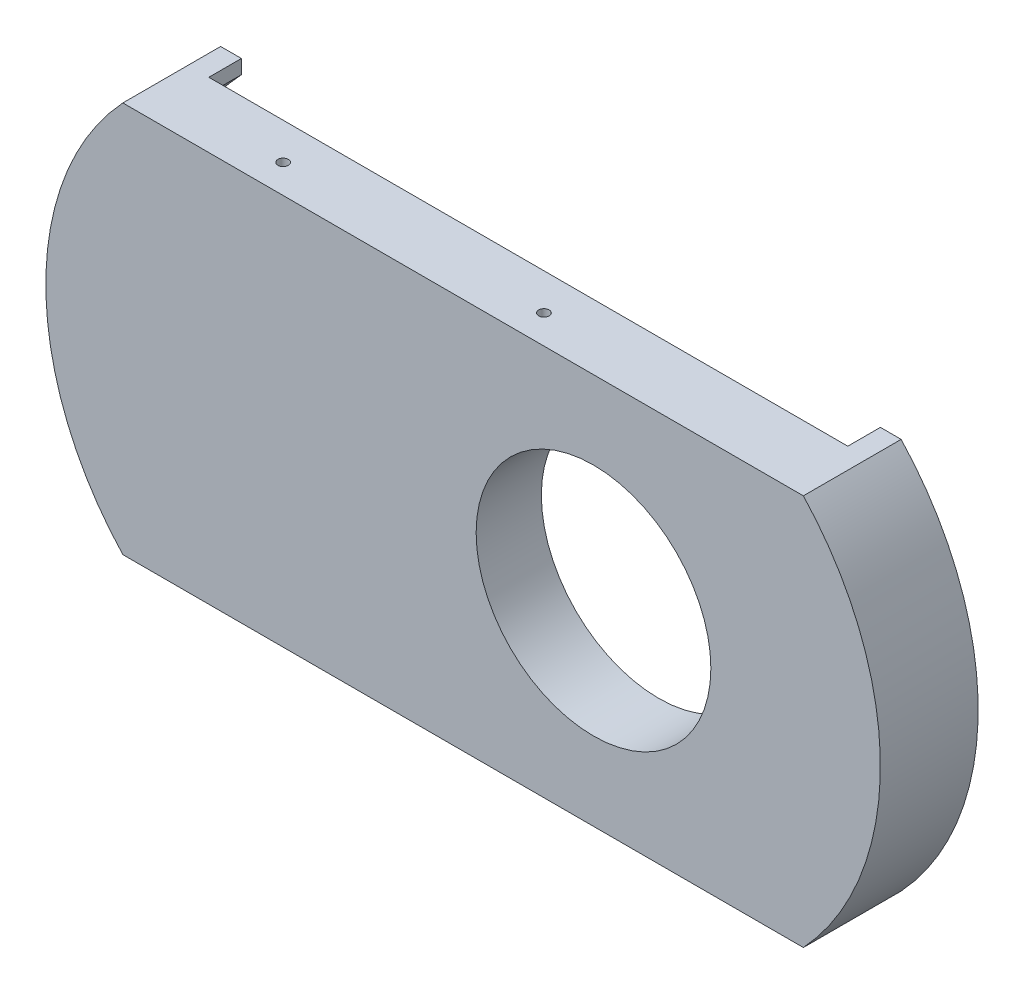
from build123d import *

# Parameters (mm, degrees)
SKETCH1_R                      = 2
BOSS_EXTRUDE1_DEPTH            = 5
SKETCH2_R                      = 8.5
CUT_EXTRUDE1_DEPTH             = 2
CUT_EXTRUDE2_REACH             = 37.693
SKETCH3_R                      = 9
BOSS_EXTRUDE2_START            = 2.5
BOSS_EXTRUDE2_DEPTH            = 2.5
SKETCH5_W                      = 49
SKETCH5_H                      = 36.444930448
CUT_EXTRUDE3_DEPTH             = 11.5
F_0_8_0_8_DIAMETER_HOLE1_D     = 0.8
F_0_8_0_8_DIAMETER_HOLE1_DEPTH = 1
F_0_8_0_8_DIAMETER_HOLE1_TIP   = 0.240344248
SKETCH8_R                      = 2
BOSS_EXTRUDE3_DEPTH            = 3
F_0_8_0_8_DIAMETER_HOLE2_D     = 0.8
F_0_8_0_8_DIAMETER_HOLE2_DEPTH = 1
F_0_8_0_8_DIAMETER_HOLE2_TIP   = 0.240344248


with BuildPart() as part:
    # Sketch1 → Boss-Extrude1 (new body)
    with BuildSketch(Plane.XY):
        with BuildLine():
            Line((-26.093476939, 15), (26.093476939, 15))
            ThreePointArc((26.093476939, 15), (32, 0), (26.093476939, -15))
            Line((26.093476939, -15), (-26.093476939, -15))
            ThreePointArc((-26.093476939, -15), (-32, 0), (-26.093476939, 15))
        make_face()
        with Locations((-10, 0)):
            Circle(SKETCH1_R, mode=Mode.SUBTRACT)
        with Locations((10, 0)):
            Circle(SKETCH1_R, mode=Mode.SUBTRACT)
    extrude(amount=BOSS_EXTRUDE1_DEPTH)

    # Sketch2 → Cut-Extrude1 (cut)
    with BuildSketch(Plane(origin=(0, 0, 0), x_dir=(-1, 0, 0), z_dir=(0, 0, -1))):
        with Locations((10, 0)):
            Circle(SKETCH2_R)
    extrude(amount=-CUT_EXTRUDE1_DEPTH, mode=Mode.SUBTRACT)

    # Sketch3 → Cut-Extrude2 (cut, up to next)
    with BuildSketch(Plane(origin=(0, 0, 0), x_dir=(-1, 0, 0), z_dir=(0, 0, -1)), mode=Mode.PRIVATE) as cut_extrude2_sk1:
        with Locations((-10, 0)):
            Circle(SKETCH3_R)
    cut_extrude2_tool1 = extrude(cut_extrude2_sk1.sketch, amount=-CUT_EXTRUDE2_REACH, mode=Mode.PRIVATE) & part.part
    add(cut_extrude2_tool1.solids().sort_by_distance((10, 0, 0))[0], mode=Mode.SUBTRACT)

    # Sketch4 → Boss-Extrude2 (add)
    with BuildSketch(Plane(origin=(0, 0, 0), x_dir=(-1, 0, 0), z_dir=(0, 0, -1)).offset(BOSS_EXTRUDE2_START)):
        with BuildLine():
            ThreePointArc((26.093476939, -15), (32, 0), (26.093476939, 15))
            Line((26.093476939, 15), (23.379461873, 15))
            ThreePointArc((23.379461873, 15), (30.1, 0), (23.379461873, -15))
            Line((23.379461873, -15), (26.093476939, -15))
        make_face()
        with BuildLine():
            ThreePointArc((-26.093476939, 15), (-32, 0), (-26.093476939, -15))
            Line((-26.093476939, -15), (-23.379461873, -15))
            ThreePointArc((-23.379461873, -15), (-30.1, 0), (-23.379461873, 15))
            Line((-23.379461873, 15), (-26.093476939, 15))
        make_face()
    extrude(amount=-BOSS_EXTRUDE2_DEPTH)

    # Sketch5 → Cut-Extrude3 (cut)
    with BuildSketch(Plane(origin=(0, 0, 0), x_dir=(-1, 0, 0), z_dir=(0, 0, -1))):
        Rectangle(SKETCH5_W, SKETCH5_H)
    extrude(amount=CUT_EXTRUDE3_DEPTH, mode=Mode.SUBTRACT)

    # Ø0.8 (0.8) Diameter Hole1
    with Locations(Plane(origin=(1, 12.5, 0), x_dir=(-1, 0, 0), z_dir=(0, 0, -1))):
        with Locations((0, 0), (-20, 0)):
            Hole(F_0_8_0_8_DIAMETER_HOLE1_D / 2, depth=F_0_8_0_8_DIAMETER_HOLE1_DEPTH)
            with Locations((0, 0, -(F_0_8_0_8_DIAMETER_HOLE1_DEPTH + F_0_8_0_8_DIAMETER_HOLE1_TIP / 2))):  # 118° drill point
                Cone(0, F_0_8_0_8_DIAMETER_HOLE1_D / 2, F_0_8_0_8_DIAMETER_HOLE1_TIP, mode=Mode.SUBTRACT)

    # Sketch8 → Boss-Extrude3 (add)
    with BuildSketch(Plane(origin=(0, 0, 2), x_dir=(-1, 0, 0), z_dir=(0, 0, -1))):
        with Locations((10, 0)):
            Circle(SKETCH8_R)
    extrude(amount=-BOSS_EXTRUDE3_DEPTH)

    # Ø0.8 (0.8) Diameter Hole2
    with Locations(Plane(origin=(-16, 15, 2.8), x_dir=(1, 0, 0), z_dir=(0, 1, 0))):
        with Locations((0, 0), (20, 0)):
            Hole(F_0_8_0_8_DIAMETER_HOLE2_D / 2, depth=F_0_8_0_8_DIAMETER_HOLE2_DEPTH)
            with Locations((0, 0, -(F_0_8_0_8_DIAMETER_HOLE2_DEPTH + F_0_8_0_8_DIAMETER_HOLE2_TIP / 2))):  # 118° drill point
                Cone(0, F_0_8_0_8_DIAMETER_HOLE2_D / 2, F_0_8_0_8_DIAMETER_HOLE2_TIP, mode=Mode.SUBTRACT)


solid = part.part
